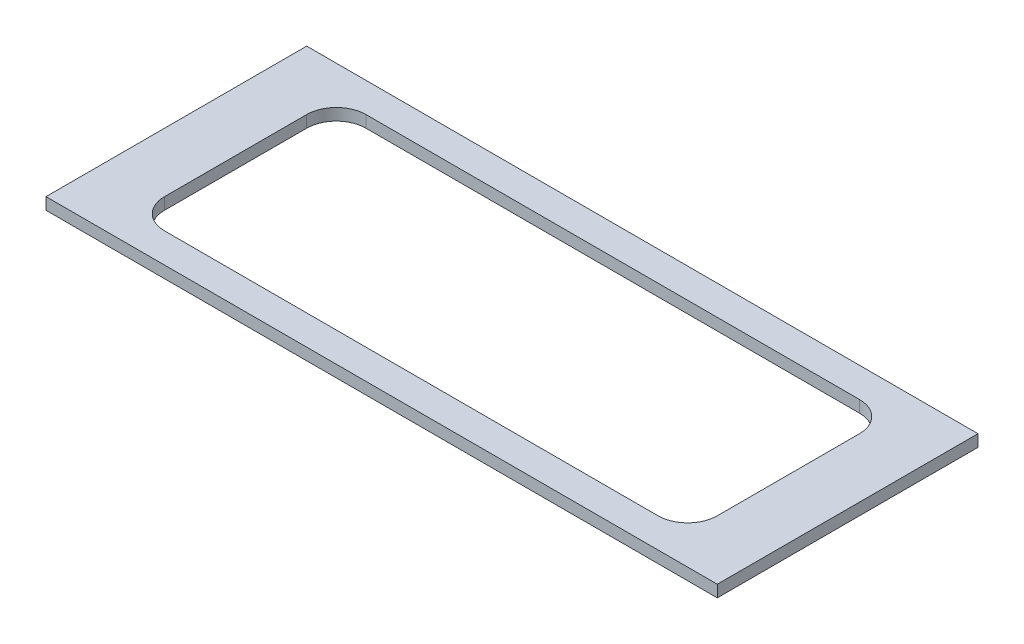
SolidWorks part; units mm, degrees
ref_plane "前视基准面" through (0, 0, 0) normal (0, 0, 1) x (1, 0, 0)
ref_plane "上视基准面" through (0, 0, 0) normal (0, 1, 0) x (1, 0, 0)
ref_plane "右视基准面" through (0, 0, 0) normal (1, 0, 0) x (0, 0, -1)
sketch "草图1" plane through (0, 0, 0) normal (0, 1, 0) x (1, 0, 0)
  line L1 (-1133, -440) -> (1133, -440)
  line L2 (-1133, -440) -> (-1133, 440)
  line L3 (-1133, 440) -> (1133, 440)
  line L4 (1133, -440) -> (1133, 440)
  line L5 (-1133, -440) -> (1133, 440) construction
  line L6 (-1133, 440) -> (1133, -440) construction
  point P0 (0, 0)
  dimension "D1" = 2266
  dimension "D2" = 880
extrude "凸台-拉伸1" add sketch "草图1" along normal blind 40
sketch "草图2" plane through (0, 0, 0) normal (0, -1, 0) x (1, 0, 0)
  line L0 (1133, 440) -> (1133, -440) construction
  line L1 (-933, 340) -> (933, 340)
  line L2 (-933, 340) -> (-933, -340)
  line L3 (-933, -340) -> (933, -340)
  line L4 (933, 340) -> (933, -340)
  line L5 (-933, 340) -> (933, -340) construction
  line L6 (-933, -340) -> (933, 340) construction
  line L7 (-1133, -440) -> (-1133, 440) construction
  line L8 (1133, -440) -> (-1133, -440) construction
  line L9 (-1133, 440) -> (1133, 440) construction
  dimension "D1" = 200
  dimension "D2" = 200
  dimension "D3" = 100
  dimension "D4" = 100
extrude "切除-拉伸1" cut sketch "草图2" against normal through all
fillet "圆角1" radius 100 4 edges at (-933, 20, -340) (-933, 20, 340) (933, 20, -340) (933, 20, 340)
